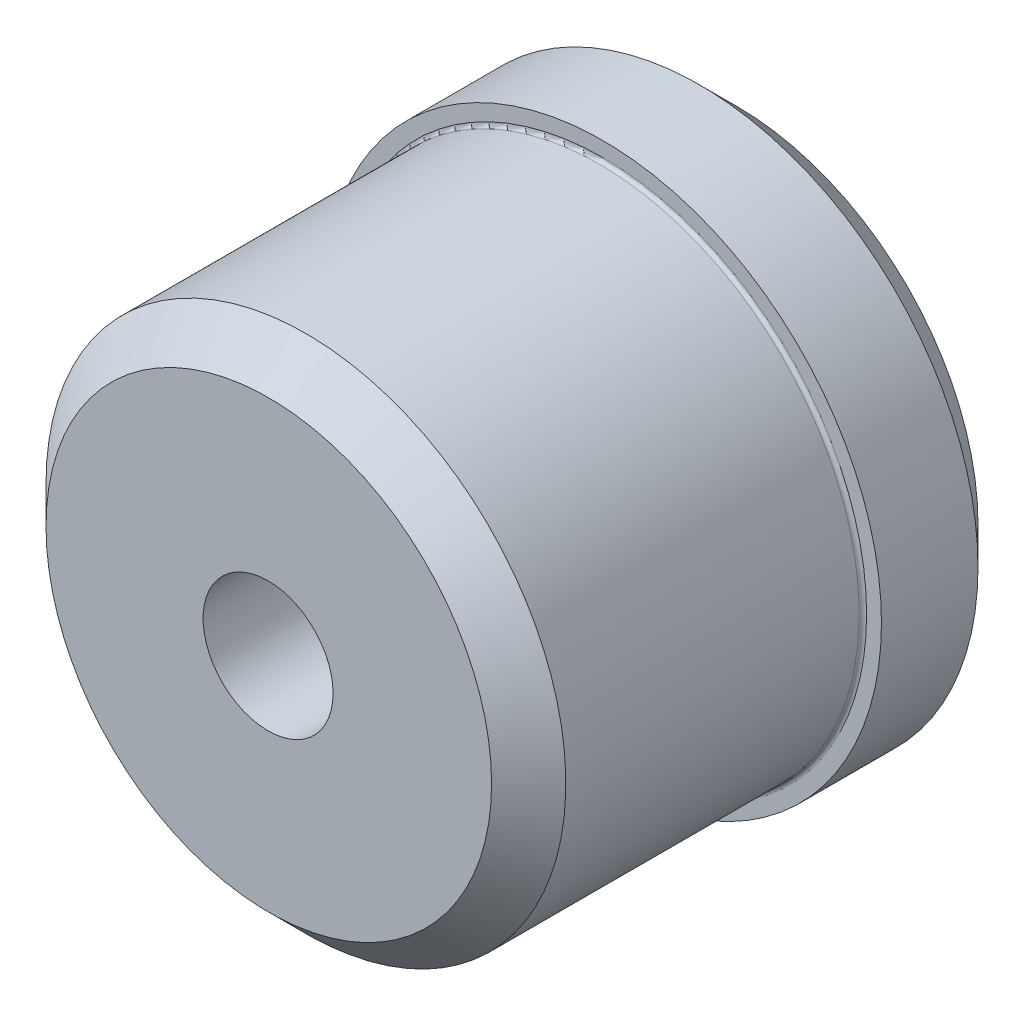
from build123d import *

# Parameters (mm, degrees)
SKETCH_1_R          = 35
EXTRUDE_1_DEPTH     = 45
SKETCH_5_R          = 37.5
EXTRUDE_2_DEPTH     = 18
CHAMFER_1_SIZE      = 5
HOLE_WIZARD_M20_1_D = 17.5
FILLET_1_R          = 0.5


with BuildPart() as part:
    # 草图1 → 凸台-拉伸1 (new body)
    with BuildSketch(Plane.XY):
        with Locations(Location((0, 0, 0), (0, 0, 180))):
            Circle(SKETCH_1_R)
    extrude(amount=EXTRUDE_1_DEPTH)

    # 草图5 → 凸台-拉伸2 (add)
    with BuildSketch(Plane(origin=(0, 0, 0), x_dir=(-1, 0, 0), z_dir=(0, 0, -1))):
        Circle(SKETCH_5_R)
    extrude(amount=EXTRUDE_2_DEPTH)

    # 倒角1
    chamfer_1_edges = [part.edges().sort_by_distance(p)[0] for p in [
        (35, 0, 45),
        (37.5, 0, -18),
    ]]
    chamfer(chamfer_1_edges, length=CHAMFER_1_SIZE)

    # M20 螺纹孔1 (through all)
    with Locations(Plane(origin=(-0.093425474, -0.140138211, 45), x_dir=(1, 0, 0), z_dir=(0, 0, 1))):
        with Locations((0, 0)):
            Hole(HOLE_WIZARD_M20_1_D / 2)

    # 圆角1
    fillet_1_edges = [part.edges().sort_by_distance(p)[0] for p in [
        (35, 0, 0),
    ]]
    fillet(fillet_1_edges, radius=FILLET_1_R)


solid = part.part
